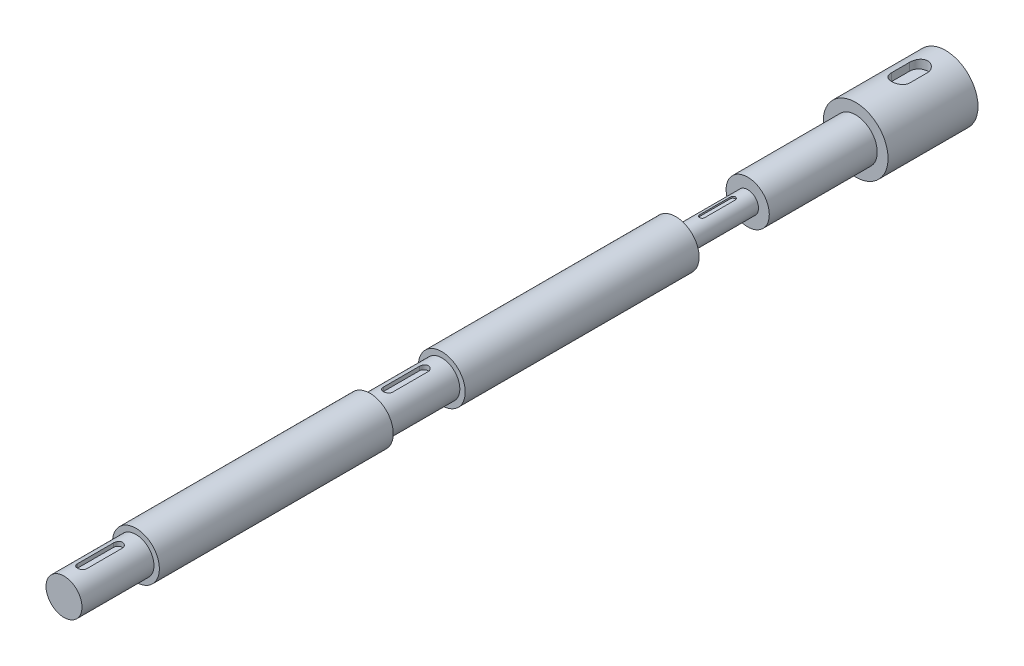
SolidWorks part; units mm, degrees
ref_plane "Front Plane" through (0, 0, 0) normal (0, 0, 1) x (1, 0, 0)
ref_plane "Top Plane" through (0, 0, 0) normal (0, 1, 0) x (1, 0, 0)
ref_plane "Right Plane" through (0, 0, 0) normal (1, 0, 0) x (0, 0, -1)
sketch "Sketch1" plane through (0, 0, 0) normal (0, 0, 1) x (1, 0, 0)
  circle A0 centre (0, 0) radius 18
  dimension "D1" = 36
extrude "Boss-Extrude2" add sketch "Sketch1" along normal mid plane 50
sketch "Sketch2" plane through (0, 0, 25) normal (0, 0, 1) x (1, 0, 0)
  circle A0 centre (0, 0) radius 18
  dimension "D1" = 36
sketch "Sketch6" plane through (0, 0, 25) normal (0, 0, 1) x (1, 0, 0)
  circle A0 centre (0, 0) radius 12
  dimension "D1" = 24
extrude "Boss-Extrude6" add sketch "Sketch6" along normal blind 60
sketch "Sketch7" plane through (0, 0, 85) normal (0, 0, 1) x (1, 0, 0)
  circle A0 centre (0, 0) radius 6
  dimension "D1" = 12
extrude "Boss-Extrude7" add sketch "Sketch7" along normal blind 30
ref_plane "Plane1" through (0, 13, 0) normal (0, 1, 0) x (-1, 0, 0)
ref_plane "Plane2" through (0, 5, 0) normal (0, 1, 0) x (-1, 0, 0)
sketch "Sketch11" plane through (0, 13, 0) normal (0, 1, 0) x (-1, 0, 0)
  line L0 (0, 21.0658) -> (0, -16.0286) construction
  line L1 (-5, 0) -> (-5, -10)
  line L2 (5, -10) -> (5, 0)
  line L3 (-18, -25) -> (18, -25) construction
  arc A0 (-5, -10) -> (5, -10) centre (0, -10) ccw
  arc A1 (5, 0) -> (-5, 0) centre (0, 0) ccw
  dimension "D1" = 10
  dimension "D2" = 10
  dimension "D3" = 15
extrude "Cut-Extrude3" cut sketch "Sketch11" along normal blind 10
sketch "Sketch12" plane through (0, 5, 0) normal (0, 1, 0) x (-1, 0, 0)
  line L0 (0, 91.453) -> (0, -9.6909) construction
  line L1 (-1.4, 110.5) -> (-1.4, 93.3)
  line L2 (1.4, 93.3) -> (1.4, 110.5)
  line L3 (6, 115) -> (-6, 115) construction
  arc A0 (-1.4, 93.3) -> (1.4, 93.3) centre (0, 93.3) ccw
  arc A1 (1.4, 110.5) -> (-1.4, 110.5) centre (0, 110.5) ccw
  dimension "D1" = 2.8
  dimension "D2" = 17.2
  dimension "D3" = 4.5
extrude "Cut-Extrude4" cut sketch "Sketch12" along normal blind 5
sketch "Sketch13" plane through (0, 0, 0) normal (0, 1, 0) x (1, 0, 0)
  line L0 (0, -75.1614) -> (0, -496.9801) construction
  line L1 (-6, -125) -> (-13, -125)
  line L2 (-10, -465) -> (0, -465)
  line L3 (-13, -125) -> (-13, -255)
  line L4 (-13, -255) -> (-10, -255)
  line L5 (-10, -255) -> (-10, -295)
  line L6 (0, -115) -> (-6, -115)
  line L7 (-6, -115) -> (-6, -125)
  line L8 (-6, -125) -> (-13, -125)
  line L9 (-13, -295) -> (-13, -425)
  line L10 (-10, -295) -> (-13, -295)
  line L11 (-10, -425) -> (-10, -465)
  line L12 (-10, -425) -> (-13, -425)
  line L13 (-10, -295) -> (-13, -295)
  dimension "D1" = 13
  dimension "D2" = 130
  dimension "D3" = 20
  dimension "D4" = 40
  dimension "D5" = 10
revolve "Revolve1" add sketch "Sketch13" angle 360 about L0
ref_plane "Plane3" through (0, 10, 0) normal (0, 1, 0) x (1, 0, 0)
sketch "Sketch14" plane through (0, 10, 0) normal (0, 1, 0) x (1, 0, 0)
  line L0 (0, -201.8318) -> (0, -295) construction
  line L1 (13, -295) -> (-13, -295) construction
sketch "Sketch16" plane through (0, 10, 0) normal (0, 1, 0) x (1, 0, 0)
  line L1 (0, -265) -> (0, -285) construction
  line L2 (2.5, -265) -> (2.5, -285)
  line L3 (-2.5, -265) -> (-2.5, -285)
  line L4 (10, -295) -> (-10, -295) construction
  arc A0 (2.5, -265) -> (-2.5, -265) centre (0, -265) ccw
  arc A1 (-2.5, -285) -> (2.5, -285) centre (0, -285) ccw
  point P0 (0, -275)
  dimension "D3" = 2.5
  dimension "D1" = 20
  dimension "D2" = 20
extrude "Cut-Extrude5" cut sketch "Sketch16" against normal blind 2.5
ref_plane "Plane4" through (0, 10, 0) normal (0, 1, 0) x (1, 0, 0)
sketch "Sketch17" plane through (0, 10, 0) normal (0, 1, 0) x (1, 0, 0)
  line L0 (0, -329.34) -> (0, -359.5884) construction
  line L1 (0, -435) -> (0, -455) construction
  line L2 (2.5, -435) -> (2.5, -455)
  line L3 (-2.5, -435) -> (-2.5, -455)
  line L4 (-10, -465) -> (10, -465) construction
  arc A0 (2.5, -435) -> (-2.5, -435) centre (0, -435) ccw
  arc A1 (-2.5, -455) -> (2.5, -455) centre (0, -455) ccw
  point P5 (0, -445)
  dimension "D3" = 2.5
  dimension "D1" = 20
  dimension "D2" = 20
extrude "Cut-Extrude6" cut sketch "Sketch17" against normal blind 2.5
